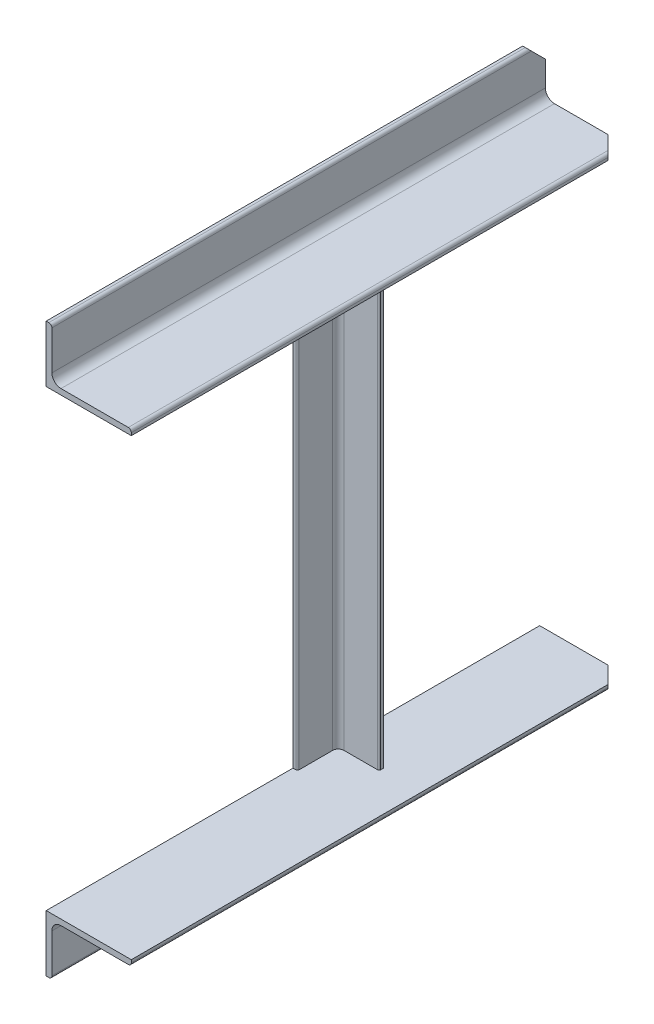
SolidWorks part; units mm, degrees
material "SPCC冷轧板喷塑"
ref_plane "前视基准面" through (0, 0, 0) normal (0, 0, 1) x (1, 0, 0)
ref_plane "上视基准面" through (0, 0, 0) normal (0, 1, 0) x (1, 0, 0)
ref_plane "右视基准面" through (0, 0, 0) normal (1, 0, 0) x (0, 0, -1)
other "Configuration Table"
sketch "草图1" plane through (0, 0, 0) normal (1, 0, 0) x (0, 0, -1)
  line L0 (-217.5, 0) -> (217.5, 0)
  point P5 (0, 0)
  dimension "D1" = 435
other "Gbt706-2008 热轧不等边角钢 075×50×5(1)"
ref_plane "基准面1" through (0, 0, 217.5) normal (0, 0, -1) x (0, 1, 0)
sketch "Sketch12" plane through (0, 0, 217.5) normal (0, 0, -1) x (0, 1, 0)
  line L0 (0, 0) -> (0, 75)
  line L1 (0, 37.5) -> (5, 37.5) construction
  line L2 (5, 72.3333) -> (5, 13)
  line L3 (13, 5) -> (47.3333, 5)
  line L4 (25, 5) -> (25, 0) construction
  line L5 (50, 0) -> (0, 0)
  line L6 (0, 75) -> (2.3333, 75)
  line L7 (50, 0) -> (50, 2.3333)
  arc A0 (50, 2.3333) -> (47.3333, 5) centre (47.3333, 2.3333) ccw
  arc A1 (2.3333, 75) -> (5, 72.3333) centre (2.3333, 72.3333) cw
  arc A2 (13, 5) -> (5, 13) centre (13, 13) cw
  point P10 (25, 0)
  point P14 (0, 37.5)
  point P15 (5, 37.5)
  point P16 (25, 5)
  point P21 (0, 0)
ref_plane "基准面2" through (0, -200, 0) normal (0, -1, 0) x (-1, 0, 0)
sketch "草图2" plane through (0, 0, 0) normal (-1, 0, 0) x (0, 0, 1)
  line L0 (-217.5, 35) -> (-202.5, 50)
  line L1 (-217.5, 0) -> (-217.5, 50) construction
  line L2 (-217.5, 50) -> (217.5, 50) construction
  dimension "D1" = 15
  dimension "D2" = 15
extrude "切除-拉伸1" cut sketch "草图2" against normal blind 10 and the other way through all
sketch "草图3" plane through (0, 0, 0) normal (0, -1, 0) x (1, 0, 0)
  line L0 (60, -217.5) -> (75, -202.5)
  line L2 (75, -217.5) -> (75, 217.5) construction
  line L3 (75, -217.5) -> (0, -217.5) construction
  dimension "D1" = 15
  dimension "D2" = 15
extrude "切除-拉伸2" cut sketch "草图3" against normal blind 10 and the other way through all flip side to cut
mirror "镜向2" about plane through (0, -200, 0) normal (0, -1, 0) of bodies 110
sketch "草图5" plane through (0, 0, 0) normal (-1, 0, 0) x (0, 0, 1)
  line L0 (0, 0) -> (0, -400)
  line L1 (-217.5, -400) -> (217.5, -400) construction
other "Gbt706-2008 热轧等边角钢 040×4(1)"
ref_plane "基准面3" through (0, 0, -40) normal (0, 1, 0) x (0, 0, 1)
sketch "Sketch15" plane through (0, 0, -40) normal (0, 1, 0) x (0, 0, 1)
  line L0 (0, 0) -> (0, 40)
  line L1 (0, 20) -> (4, 20) construction
  line L2 (4, 38.6667) -> (4, 9)
  line L3 (9, 4) -> (38.6667, 4)
  line L4 (20, 4) -> (20, 0) construction
  line L5 (40, 0) -> (0, 0)
  line L6 (0, 40) -> (2.6667, 40)
  line L7 (40, 0) -> (40, 2.6667)
  arc A0 (40, 2.6667) -> (38.6667, 4) centre (38.6667, 2.6667) ccw
  arc A1 (2.6667, 40) -> (4, 38.6667) centre (2.6667, 38.6667) cw
  arc A2 (9, 4) -> (4, 9) centre (9, 9) cw
  point P10 (20, 0)
  point P14 (0, 20)
  point P15 (4, 20)
  point P16 (20, 4)
  point P17 (4, 40)
  point P18 (40, 4)
  point P21 (40, 4)
  point P24 (4, 40)
  point P25 (0, 0)
equation "\"D2@Sketch12\"= \"Radius_1@Sketch12\" / 3"
equation "\"D4@Sketch12\"= \"D1@Sketch12\""
equation "\"D2@Sketch15\"= \"D1@Sketch15\" / 3"
